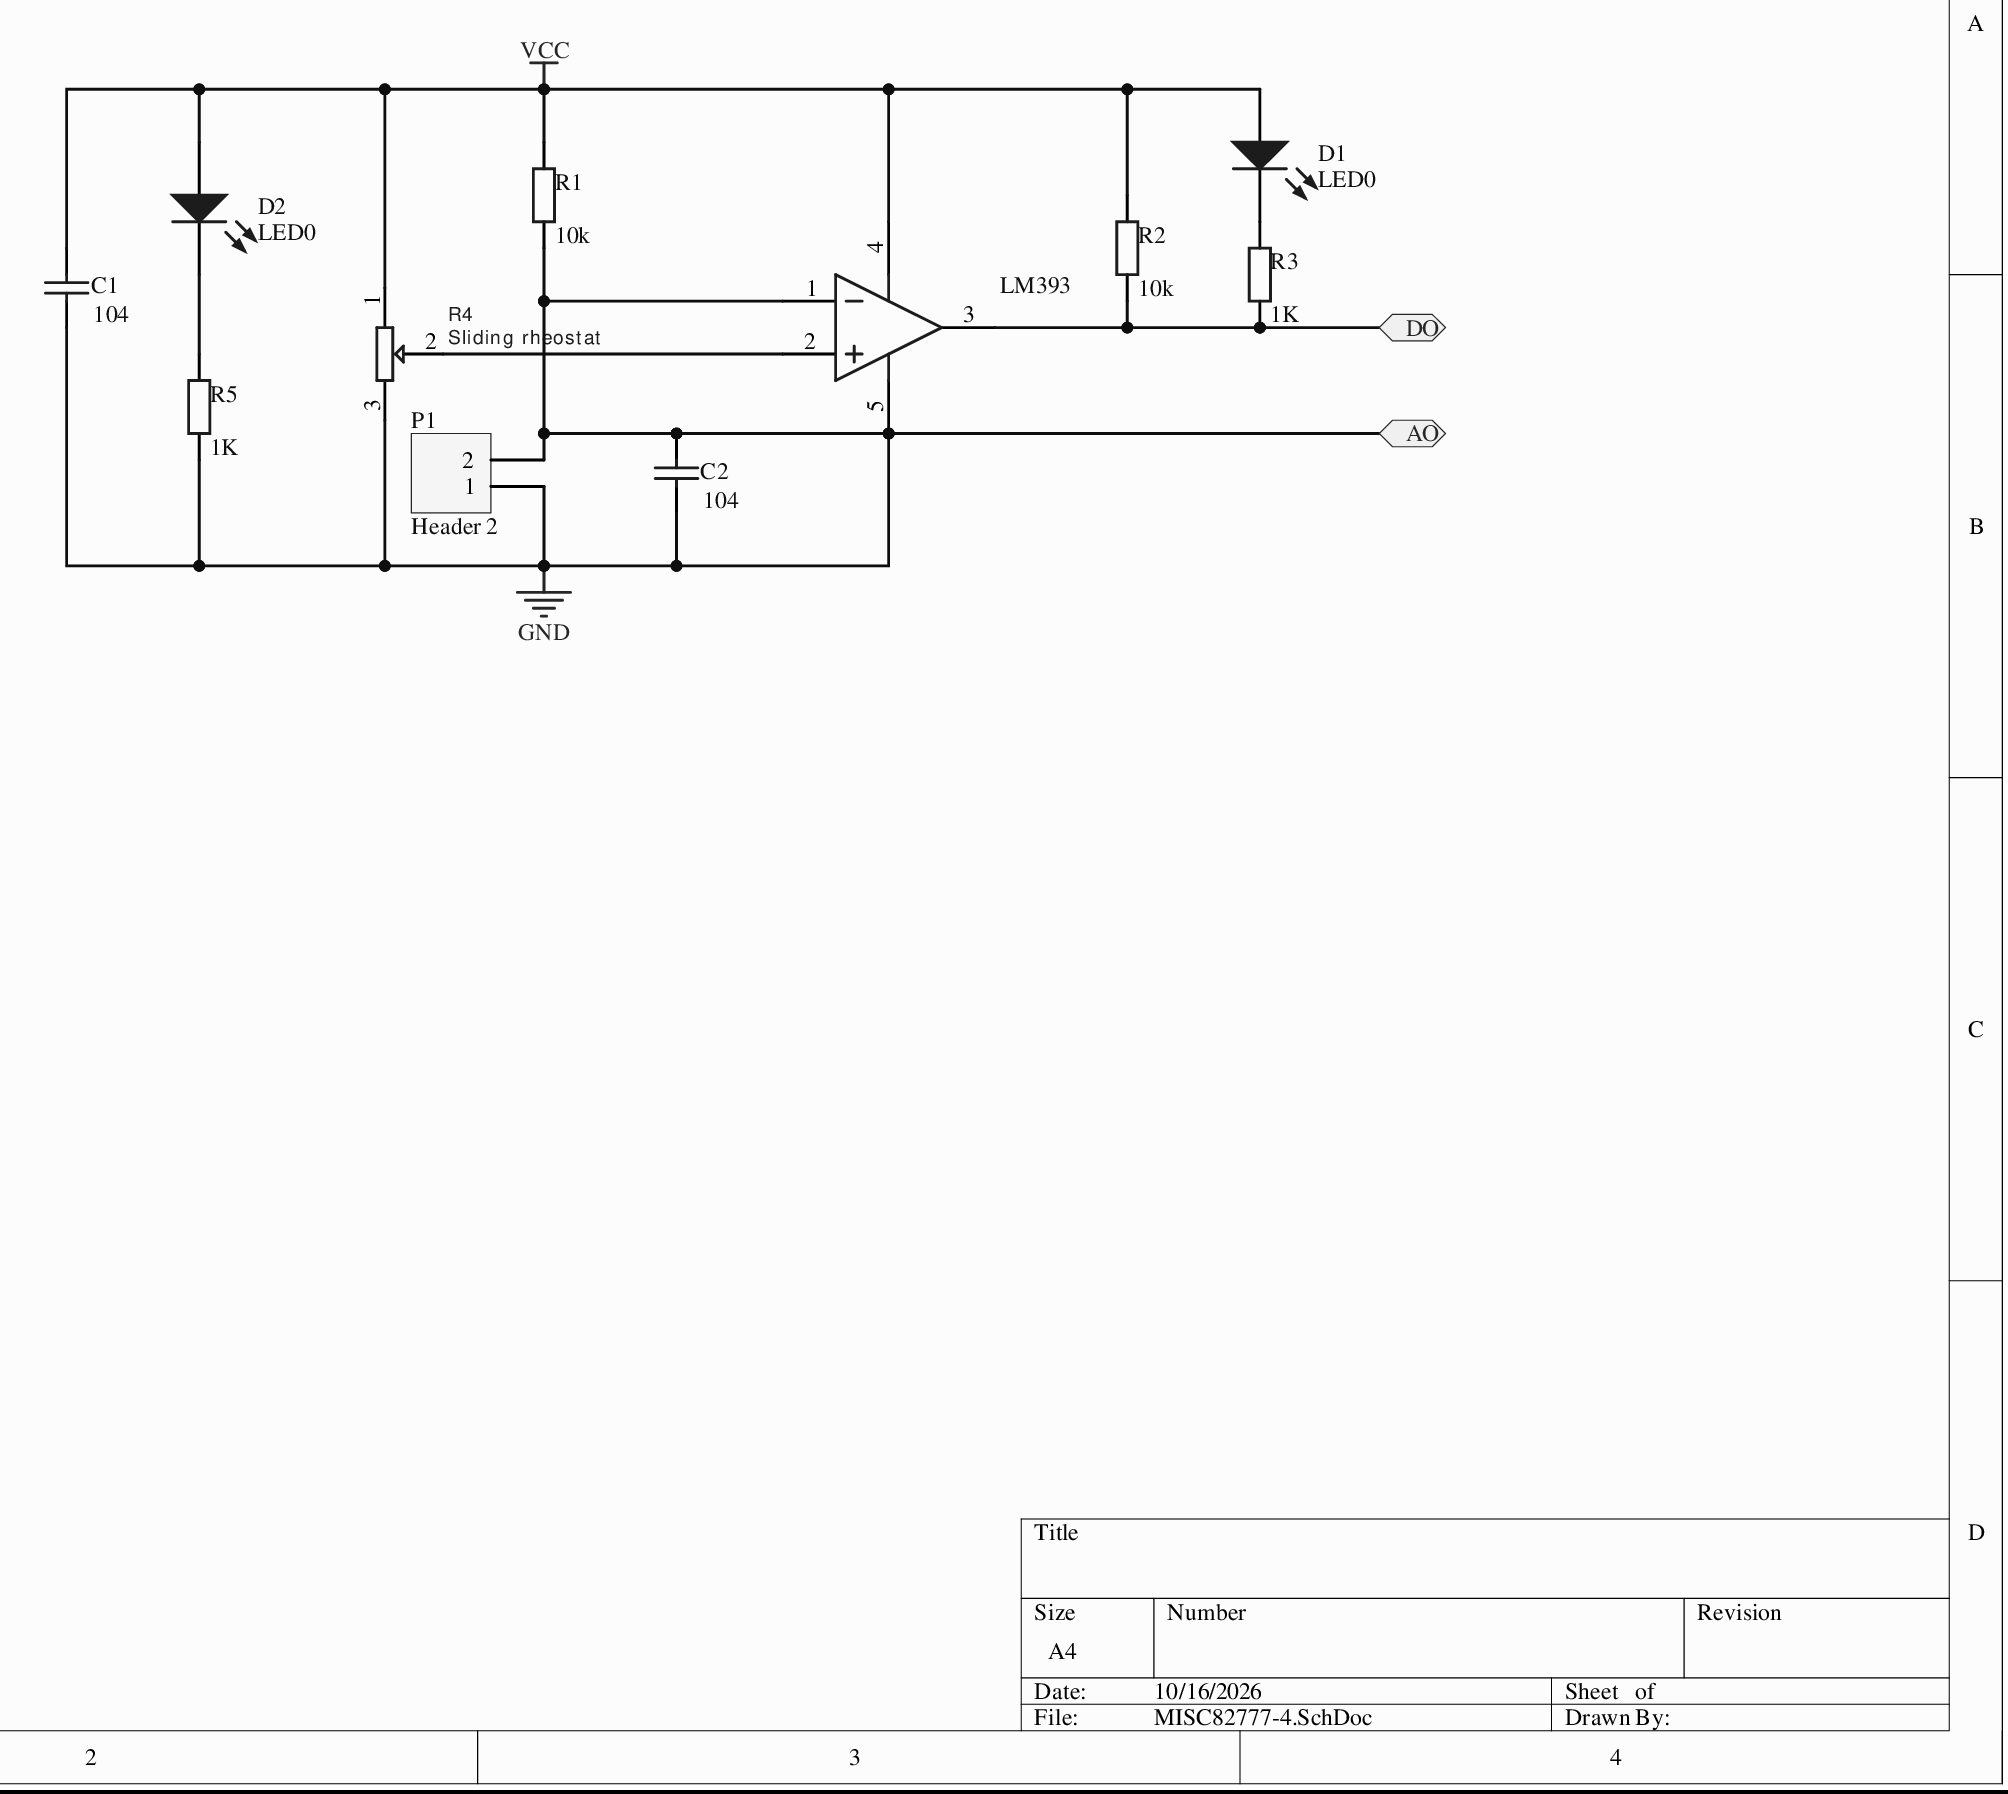
[diagram p0: MISC82777-4.SchDoc]
# Altium project MISC82777-7.PrjPcb
1 sheet, 11 parts. Net scope: flat (ports and power ports of the same name join across sheets).
Board file: MISC82777.PcbDoc

## Sheet MISC82777-4.SchDoc
size A4

### Parts
C1  value 104  [RAD-0.3]  (hidden comment: Cap)
C2  value 104  [RAD-0.3]  (hidden comment: Cap)
D1  LED0  [LED-0]
D2  LED0  [LED-0]
P1  Header 2  [HDR1X2]
R1  value 10k  [AXIAL-0.4]  (hidden comment: Res2)
R2  value 10k  [AXIAL-0.4]  (hidden comment: Res2)
R3  value 1K  [AXIAL-0.4]  (hidden comment: Res2)
R4  Sliding rheostat  [滑动变阻器]
R5  value 1K  [AXIAL-0.4]  (hidden comment: Res2)
U1  LM393  [626-05]  (part A of 2)

### Ports
AO (bidir), DO (bidir)

### Nets
GND: C1.1 C2.1 C2.2 P1.1 P1.2 R1.1 R4.3 R5.1 U1.1(IN-) U1.5(GND) ; port AO
VCC: C1.2 D1.1(A) D2.1(A) R1.2 R2.2 R4.1 U1.4(V+)
NetD1_2: D1.2(K) R3.2
NetD2_2: D2.2(K) R5.2
NetR2_1: R2.1 R3.1 U1.3(OUT) ; port DO
NetR4_2: R4.2 U1.2(IN+)

### Library data of the parts
C1 C2 = Cap: Capacitor; Published: 8-Jun-2000; LatestRevisionDate: 17-Jul-2002; LatestRevisionNote: Re-released for DXP Platform.; PackageReference: RAD-0.3; PackageDescription: Radial Cap, Thru-Hole; 2 Leads; 0.3 in Pin Spacing; Publisher: Altium Limited
D1 D2 = LED0: Typical INFRARED GaAs LED; Published: 8-Jun-2000; LatestRevisionDate: 08-Jul-2005; LatestRevisionNote: Mech Layer 1 removed.; PackageReference: LED-0; PackageDescription: LED; 2 Leads; Publisher: Altium Limited
P1 = Header 2: Header, 2-Pin; LatestRevisionDate: 17-Jul-2002; LatestRevisionNote: Re-released for DXP Platform.; Publisher: Altium Limited
R1-R3 R5 = Res2: Resistor; Published: 8-Jun-2000; LatestRevisionDate: 17-Jul-2002; LatestRevisionNote: Re-released for DXP Platform.; PackageReference: AXIAL-0.4; PackageDescription: Axial Device, Thru-Hole; 2 Leads; 0.4 in Pin Spacing; Publisher: Altium Limited
R4 = 滑动变阻器
U1 = LM393N: Dual Comparator; Published: 17-Jul-2002; LatestRevisionDate: 06-Jun-2005; LatestRevisionNote: Stylized 3D Model Added.; DatasheetVersion: 1988; PackageReference: 626-05; PackageDescription: DIP; 8 Leads; Row Spacing 7.62 mm; Pitch 2.54 mm; ComponentLink1Description: Manufacturer Link; ComponentLink1URL: http://www.onsemi.com/site/products/taxonomy/0,4438,133,00.html; Publisher: Altium Limited